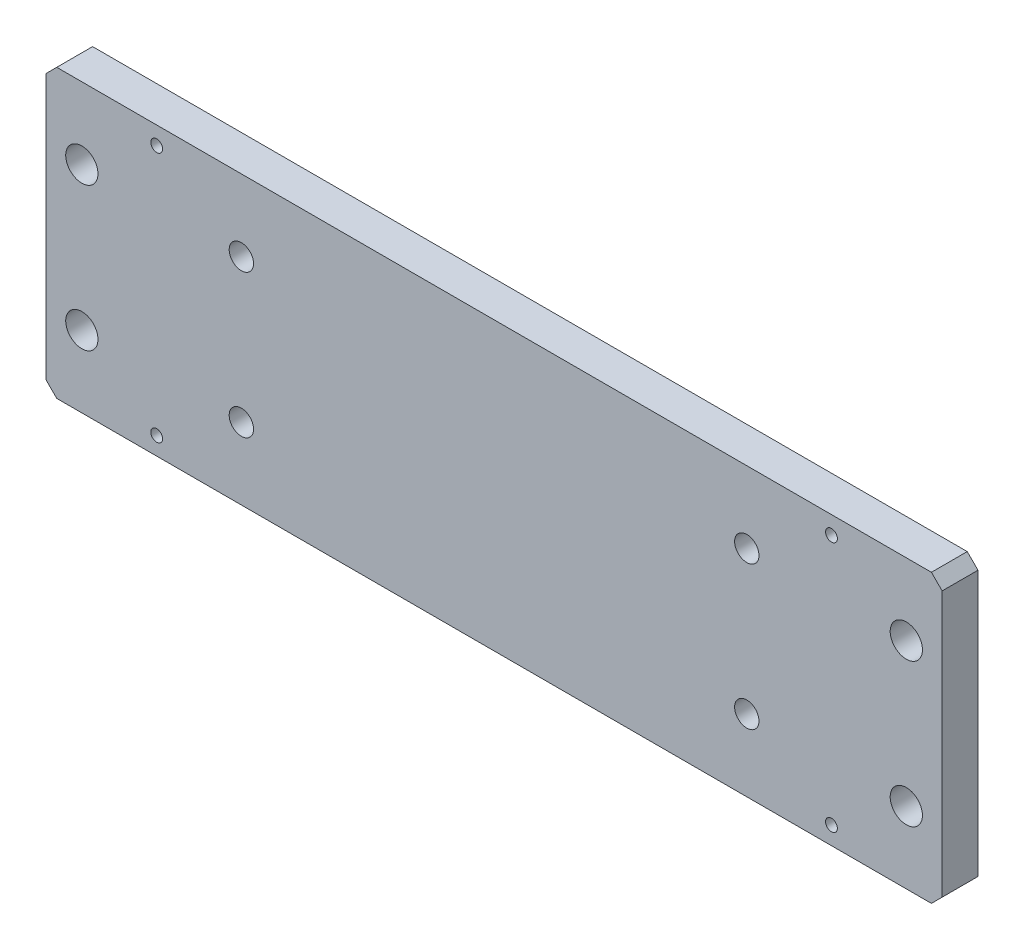
SolidWorks part; units mm, degrees
ref_plane "前视基准面" through (0, 0, 0) normal (0, 0, 1) x (1, 0, 0)
ref_plane "上视基准面" through (0, 0, 0) normal (0, 1, 0) x (1, 0, 0)
ref_plane "右视基准面" through (0, 0, 0) normal (1, 0, 0) x (0, 0, -1)
sketch "草图1" plane through (0, 0, 0) normal (0, 0, 1) x (1, 0, 0)
  line L1 (-125, 80) -> (125, 80)
  line L2 (-125, 80) -> (-125, 0)
  line L3 (-125, 0) -> (125, 0)
  line L4 (125, 80) -> (125, 0)
  dimension "D1" = 250
  dimension "D2" = 80
extrude "凸台-拉伸1" add sketch "草图1" along normal blind 10
hole_wizard "Ø9.0 (9) 直径孔1" positions "草图3" profile "草图2" hole size "Ø9.0" standard "GB" end condition through all
sketch "草图3" plane through (0, 0, 10) normal (0, 0, 1) x (1, 0, 0)
  line L0 (125, 0) -> (125, 80) construction
  line L1 (-125, 0) -> (125, 0) construction
  line L2 (125, 80) -> (-125, 80) construction
  point P0 (115, 20)
  point P2 (115, 60)
  dimension "D1" = 10
  dimension "D2" = 20
  dimension "D3" = 20
  dimension "D4" = 10
sketch "草图2" plane through (115, 20, 10) normal (1, 0, 0) x (0, -1, 0)
  line L0 (0, 0) -> (0, 10)
  line L1 (0, 10) -> (4.5, 10)
  line L2 (4.5, 10) -> (4.5, 0)
  line L5 (4.5, 0) -> (0, 0)
  line L11 (0, -6.35) -> (0, 107.95) construction
  dimension "通孔孔直径" = 9
  dimension "通孔孔深度" = 10
ref_plane "基准面1" through (0, 0, 0) normal (1, 0, 0) x (0, 0, -1)
mirror "镜向1" about plane through (0, 0, 0) normal (1, 0, 0) of "Ø9.0 (9) 直径孔1"
chamfer "倒角1" distance 3 angle 45 4 edges at (-125, 80, 5) (-125, 0, 5) (125, 0, 5) (125, 80, 5)
hole_wizard "M8 螺纹孔1" positions "草图5" profile "草图4" tap size "M8" standard "ISO" end condition through all
sketch "草图5" plane through (0, 0, 10) normal (0, 0, 1) x (1, 0, 0)
  line L0 (66, 60) -> (75, 60) construction
  line L1 (66, 47.5) -> (66, 72.5) construction
  line L2 (75, 72.5) -> (75, 47.5) construction
  line L4 (75, 20) -> (66, 20) construction
  line L5 (75, 32.5) -> (75, 7.5) construction
  line L6 (66, 7.5) -> (66, 32.5) construction
  point P0 (70.5, 60)
  point P2 (70.5, 20)
sketch "草图4" plane through (70.5, 60, 10) normal (1, 0, 0) x (0, -1, 0)
  line L0 (0, 0) -> (0, 10)
  line L1 (0, 10) -> (3.4, 10)
  line L2 (3.4, 10) -> (3.4, 0)
  line L5 (3.4, 0) -> (0, 0)
  line L11 (0, -6.35) -> (0, 107.95) construction
  dimension "通孔螺纹孔钻头直径" = 6.8
  dimension "通孔螺纹孔钻头深度" = 10
cosmetic thread "孔螺蚊线1" parameters "D2"=8
cosmetic thread "孔螺蚊线2" parameters "D2"=8
ref_plane "基准面2" through (0, 0, 0) normal (1, 0, 0) x (0, 0, -1)
mirror "镜向2" about plane through (0, 0, 0) normal (1, 0, 0) of "M8 螺纹孔1"
hole_wizard "M4 螺纹孔1" positions "草图7" profile "草图6" tap size "M4" standard "ISO" end condition through all
sketch "草图7" plane through (0, 0, 10) normal (0, 0, 1) x (1, 0, 0)
  point P0 (-94.1219, 75)
  point P3 (-94.1219, 5)
sketch "草图6" plane through (-94.1219, 75, 10) normal (1, 0, 0) x (0, -1, 0)
  line L0 (0, 0) -> (0, 10)
  line L1 (0, 10) -> (1.65, 10)
  line L2 (1.65, 10) -> (1.65, 0)
  line L5 (1.65, 0) -> (0, 0)
  line L11 (0, -6.35) -> (0, 107.95) construction
  dimension "通孔螺纹孔钻头直径" = 3.3
  dimension "通孔螺纹孔钻头深度" = 10
cosmetic thread "孔螺蚊线3" parameters "D2"=4
cosmetic thread "孔螺蚊线4" parameters "D2"=4
ref_plane "基准面3" through (0, 0, 0) normal (-1, 0, 0) x (0, 0, 1)
mirror "镜向3" about plane through (0, 0, 0) normal (-1, 0, 0) of "M4 螺纹孔1"
